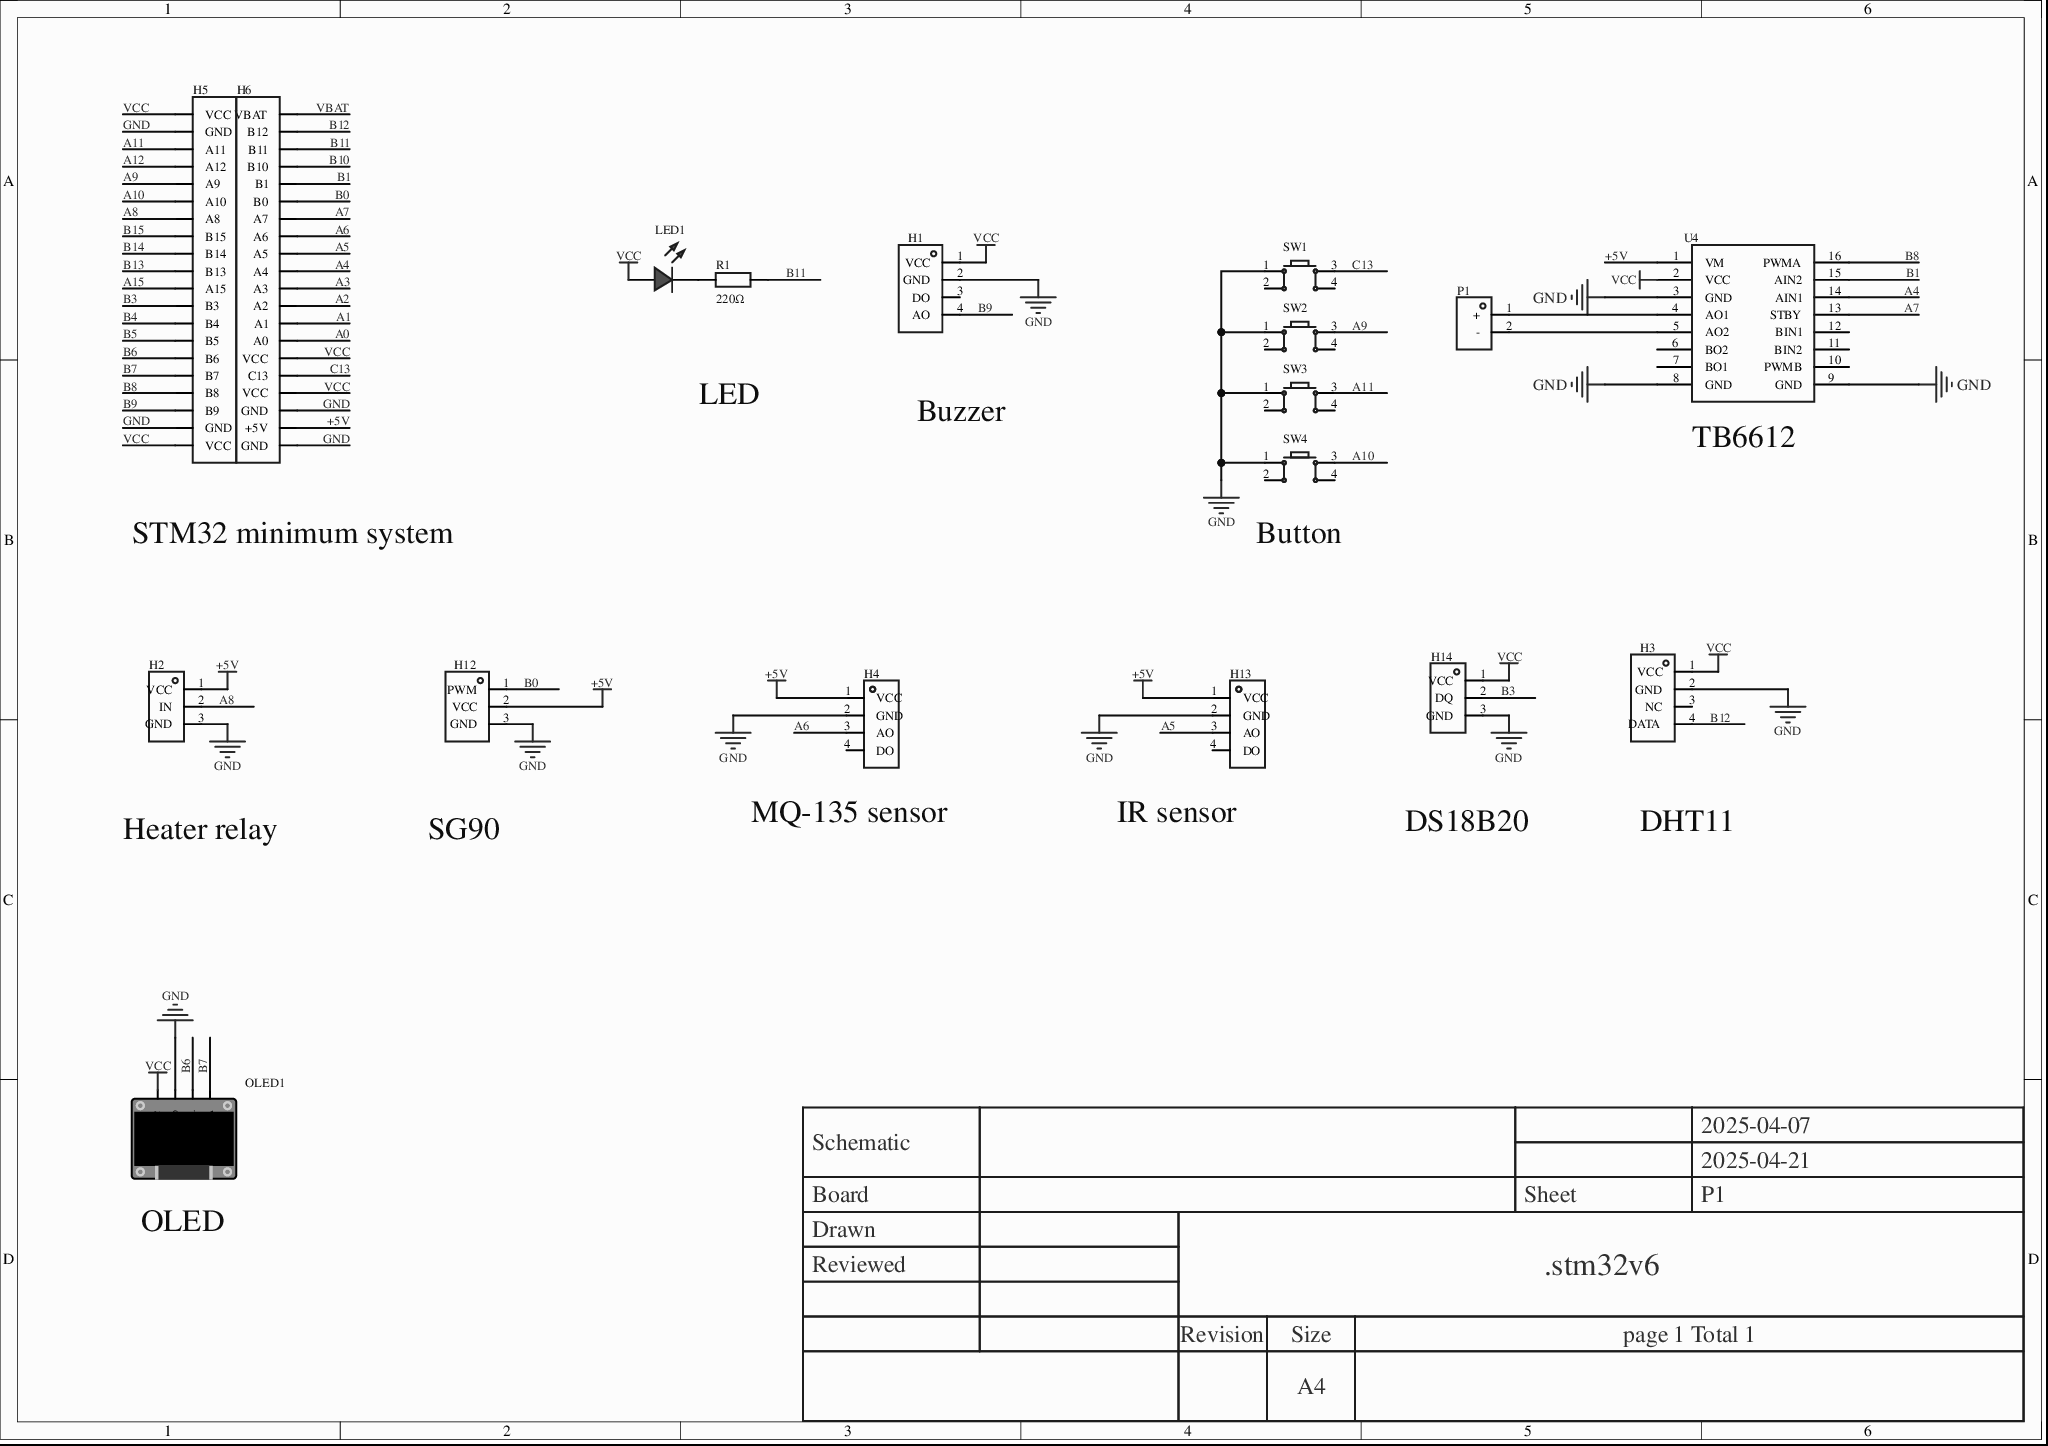
[diagram p0: MISC89119-3.schdoc]
# Altium project MISC89119-2.PrjPcb
1 sheet, 18 parts. Net scope: global (net labels, ports and power ports of the same name join across sheets).
Board file: MISC89119.pcbdoc

## Sheet MISC89119-3.schdoc
size 297 x 209 mm; Version: V1.0; @Project Name: MISC89119; @Page Count: 1; @Update Date: 2026-05-11; @Create Date: 2026-05-11; @Schematic Name: MISC89119; @Page No: 1; @Create Time: 23:22:16; @Update Time: 17:32:40; @Board Name: MISC89119

### Parts
H1  (no value)  [HDR-TH_4P-P2.54-V-F]
H2  (no value)  [HDR-TH_3P-P2.54-V-F]
H3  (no value)  [HDR-TH_4P-P2.54-V-F]
H4  (no value)  [HDR-TH_4P-P2.54-V-F]
H5  (no value)  [HDR-TH_20P-P2.54-V-F]
H6  (no value)  [HDR-TH_20P-P2.54-V-F]
H12  (no value)  [HDR-TH_3P-P2.54-V-F]
H13  (no value)  [HDR-TH_4P-P2.54-V-F]
H14  (no value)  [HDR-TH_3P-P2.54-V-F]
LED1  (no value)  [LED_TH-3mm]
OLED1  (no value)  [0.96OLED_4P]
P1  KF301-2P terminal block  [CONN-TH_XY301V-A-5.0-2P]  (value not drawn)
R1  220Ω  [Res_1/8W]
SW1  (no value)  [SW-TH_4P-L6.0-W6.0-P4.50-LS6.5]
SW2  (no value)  [SW-TH_4P-L6.0-W6.0-P4.50-LS6.5]
SW3  (no value)  [SW-TH_4P-L6.0-W6.0-P4.50-LS6.5]
SW4  (no value)  [SW-TH_4P-L6.0-W6.0-P4.50-LS6.5]
U4  (no value)  [tb6612]

### Nets
+5V: H2.1(VCC) H4.1(VCC) H6.19(+5V) H12.2(VCC) H13.1(VCC) U4.1(VM)
GND: H1.2(GND) H2.3(GND) H3.2(GND) H4.2(GND) H5.2(GND) H5.19(GND) H6.18(GND) H6.20(GND) H12.3(GND) H13.2(GND) H14.3(GND) OLED1.2(GND) SW1.1 SW2.1 SW3.1 SW4.1 U4.3(GND) U4.8(GND) U4.9(GND)
VCC: H1.1(VCC) H3.1(VCC) H5.1(VCC) H5.20(VCC) H6.15(VCC) H6.17(VCC) H14.1(VCC) LED1.1(C) OLED1.1(VCC) U4.2(VCC)
A0: H6.14(A0)
A1: H6.13(A1)
A2: H6.12(A2)
A3: H6.11(A3)
A4: H6.10(A4) U4.14(AIN1)
A5: H6.9(A5) H13.3(AO)
A6: H4.3(AO) H6.8(A6)
A7: H6.7(A7) U4.13(STBY)
A8: H2.2(IN) H5.7(A8)
A9: H5.5(A9) SW2.3
A10: H5.6(A10) SW4.3
A11: H5.3(A11) SW3.3
A12: H5.4(A12)
A15: H5.11(A15)
B0: H6.6(B0) H12.1(PWM)
B1: H6.5(B1) U4.15(AIN2)
B3: H5.12(B3) H14.2(DQ)
B4: H5.13(B4)
B5: H5.14(B5)
B6: H5.15(B6) OLED1.3(SCL)
B7: H5.16(B7) OLED1.4(SDA)
B8: H5.17(B8) U4.16(PWMA)
B9: H1.4(AO) H5.18(B9)
B10: H6.4(B10)
B11: H6.3(B11) R1.2
B12: H3.4(DATA) H6.2(B12)
B13: H5.10(B13)
B14: H5.9(B14)
B15: H5.8(B15)
C13: H6.16(C13) SW1.3
VBAT: H6.1(VBAT)
NetLED1_2: LED1.2(A) R1.1
NetP1_1: P1.1(+) U4.4(AO1)
NetP1_2: P1.2(-) U4.5(AO2)

Not connected (* = marked no-connect by the designer): H1 3(DO); H3 3(NC); H4 4(DO); H13 4(DO); SW1 2 4; SW2 2 4; SW3 2 4; SW4 2 4; U4 6(BO2) 7(BO1) 10(PWMB) 11(BIN2) 12(BIN1)

### Notes on the sheet
- LED
- Buzzer
- (near U4) TB6612
- STM32 minimum system
- (near SW4) Button
- Heater relay
- SG90
- (near H4) MQ-135 sensor
- (near H13) IR sensor
- DS18B20
- DHT11
- OLED
- 2025-04-07
- Schematic
- Board
- Sheet
- 2025-04-21
- P1
- Drawn
- Reviewed
- .stm32v6
- Revision
- Size
- A4
- page 1 Total 1

### Library data of the parts
H1 = HDR-F_2.54_1x4P: Symbol: 2.54-1*4P female_1; ConvertToPcb: yes; ModelId: d187812051054f85879fcaa51a310d8e0819f05c4eef4c71ace90d822a990e87; ModelTransform: 419.6842,98.464,0,0,0,0,0,0,-118.11; Device: HDR-F_2.54_1x4P; AddInBom: yes; SupplierPart: C2718488; Supplier Footprint: 插件; FootprintName: HDR-TH_4P-P2.54-V-F; ModelName: HDR-TH_4P-P2.54-V-F
H2 = HDR-F_2.54_1x3P: Symbol: PM254V-11-03-H85_1; 3D Model: f3b3cc5aae9641bf9e56fc160cef875b; 3D Model Transform: 299.9994,100,0,0,0,0,0,0,-118.11; ConvertToPcb: yes; ModelName: HDR2.54-F-LI-1X3P; Device: HDR-F_2.54_1x3P; Supplier Part: C541850; Supplier Footprint: 插件; FootprintName: HDR-TH_3P-P2.54-V-F; AddInBom: yes
H3 = HDR-F_2.54_1x4P: Symbol: 2.54-1*4P female_4; ConvertToPcb: yes; ModelId: d187812051054f85879fcaa51a310d8e0819f05c4eef4c71ace90d822a990e87; ModelTransform: 419.6842,98.464,0,0,0,0,0,0,-118.11; Device: HDR-F_2.54_1x4P; AddInBom: yes; SupplierPart: C2718488; Supplier Footprint: 插件; FootprintName: HDR-TH_4P-P2.54-V-F; ModelName: HDR-TH_4P-P2.54-V-F
H4 = HDR-F_2.54_1x4P: Symbol: 2.54-1*4P female_2; ConvertToPcb: yes; ModelId: d187812051054f85879fcaa51a310d8e0819f05c4eef4c71ace90d822a990e87; ModelTransform: 419.6842,98.464,0,0,0,0,0,0,-118.11; Device: HDR-F_2.54_1x4P; FootprintName: HDR-TH_4P-P2.54-V-F; AddInBom: yes; SupplierPart: C2718488; Supplier Footprint: 插件; ModelName: HDR-TH_4P-P2.54-V-F
H5 = HDR-F_2.54_1x20P: Symbol: HDR-F_2.54_1x20P_2; 3D Model: db7015f7ad9d48b8a3b1188db02e3429; 3D Model Transform: 1999.996,100,0,0,0,0,0,0,-118.11; ConvertToPcb: yes; ModelName: HDR-F-2.54_1x20; Device: HDR-F_2.54_1x20P; Supplier Part: C50984; Supplier Footprint: 插件; AddInBom: yes; FootprintName: HDR-TH_20P-P2.54-V-F
H6 = HDR-F_2.54_1x20P: Symbol: HDR-F_2.54_1x20P_3; ConvertToPcb: yes; ModelId: db7015f7ad9d48b8a3b1188db02e3429; ModelName: HDR-F-2.54_1x20; ModelTransform: 1999.996,100,0,0,0,0,0,0,-118.11; Device: HDR-F_2.54_1x20P; AddInBom: yes; SupplierPart: C50984; Supplier Footprint: 插件; FootprintName: HDR-TH_20P-P2.54-V-F
H12 = HDR-F_2.54_1x3P: Symbol: PM254V-11-03-H85_2; 3D Model: f3b3cc5aae9641bf9e56fc160cef875b; 3D Model Transform: 299.9994,100,0,0,0,0,0,0,-118.11; ConvertToPcb: yes; ModelName: HDR2.54-F-LI-1X3P; Device: HDR-F_2.54_1x3P; Supplier Part: C541850; Supplier Footprint: 插件; FootprintName: HDR-TH_3P-P2.54-V-F; AddInBom: yes
H13 = HDR-F_2.54_1x4P: Symbol: 2.54-1*4P female_3; 3D Model: d187812051054f85879fcaa51a310d8e0819f05c4eef4c71ace90d822a990e87; 3D Model Transform: 419.6842,98.464,0,0,0,0,0,0,-118.11; ConvertToPcb: yes; Device: HDR-F_2.54_1x4P; Supplier Part: C2718488; Supplier Footprint: 插件; FootprintName: HDR-TH_4P-P2.54-V-F; AddInBom: yes; ModelName: HDR-TH_4P-P2.54-V-F
H14 = HDR-F_2.54_1x3P: Symbol: PM254V-11-03-H85_3; 3D Model: f3b3cc5aae9641bf9e56fc160cef875b; 3D Model Transform: 299.9994,100,0,0,0,0,0,0,-118.11; ConvertToPcb: yes; ModelName: HDR2.54-F-LI-1X3P; Device: HDR-F_2.54_1x3P; Supplier Part: C541850; Supplier Footprint: 插件; FootprintName: HDR-TH_3P-P2.54-V-F; AddInBom: yes
LED1 = LED_TH-R_3mm: ConvertToPcb: yes; ModelId: a497c992633541038a38947cdc58012f0819f05c4eef4c71ace90d822a990e87; ModelName: LED-TH-3mm_R; ModelTransform: 141.274,153.327,0,0,0,0,-5.984,0,-137.795; Symbol: LED_TH-R; Device: LED_TH-R_3mm; AddInBom: yes; FootprintName: LED_TH-3mm; Supplier Footprint: 插件
OLED1 = 0.96OLED模块_4P: Symbol: 0.96OLED module_4P_1; Device: 0.96OLED module_4P; ConvertToPcb: yes; ModelId: 79c000fdb68d45a296c2e9bedf4f9055; ModelTransform: 1393.69792,1318.895,0,0,0,0,0,-560.079,-137.795; AddInBom: yes; FootprintName: 0.96OLED_4P; Supplier Footprint: 插件; ModelName: 0.96OLED_4P
P1 = KF301-2P接线端子: Symbol: KF301-2P terminal block_1; 3D Model: ef7ead88b0f2448d904975b26718870f; 3D Model Transform: 417.322,299.212,0,0,0,0,11.811,-7.835,-157.48; AddInBom: yes; Device: KF301-2P terminal block; LCSC Part Name: KF301-2P接线端子; Supplier Part: C9900016950; Manufacturer Part: KF301-2P接线端子; Supplier Footprint: CK301-2P; Supplier: LCSC; ConvertToPcb: yes; FootprintName: CONN-TH_XY301V-A-5.0-2P; ModelName: CONN-TH_XY301V-A-5.0-2P
R1 = Res_AXIAL-1/8W: Symbol: Resistor; ConvertToPcb: yes; ModelId: b2b5ae7ae4c642178fe0039925c86a3f0819f05c4eef4c71ace90d822a990e87; ModelName: RES-TH_BD1.8-L3.2-P7.20-D0.4; ModelTransform: 282.86,66.88,253.09,0,0,0,0,0,-191; Device: Res_AXIAL-1/8W; Value: 220Ω; AddInBom: yes; Supplier Footprint: 轴向引线; FootprintName: Res_1/8W
SW1-SW4 = Key_TH_6x6x6: 触点电流:50mA;额定电压(DC):12V;绝缘电阻:100MΩ;电路结构:单刀单掷;安装方式:直插;按钮形状:圆形按钮;按钮/盖帽颜色:黑色;作用力:260gf@±30gf;工作温度:-25℃~+70℃;引脚样式:PC引脚;开关长度:6mm;开关宽度:6mm;开关高度:6mm;带支架:否;; Symbol: Tact switch; AddInBom: yes; ModelId: 20eee248bc684ccd8cbdbb1d0d91ec6f0819f05c4eef4c71ace90d822a990e87; ModelName: SW-TH_4P-L6.0-W6.0-H5.0-LS6.5-P4.50; ModelTransform: 236.22,323.03,0,90,0,0,0,0,-137.795; Device: Key_TH_6x6x6; FootprintName: SW-TH_4P-L6.0-W6.0-P4.50-LS6.5; ConvertToPcb: yes; Supplier Footprint: 插件
U4 = tb6612: AddInBom: yes; Symbol: tb6612; Device: tb6612; JLCPCB Part Class: Extended library; ConvertToPcb: yes; FootprintName: tb6612